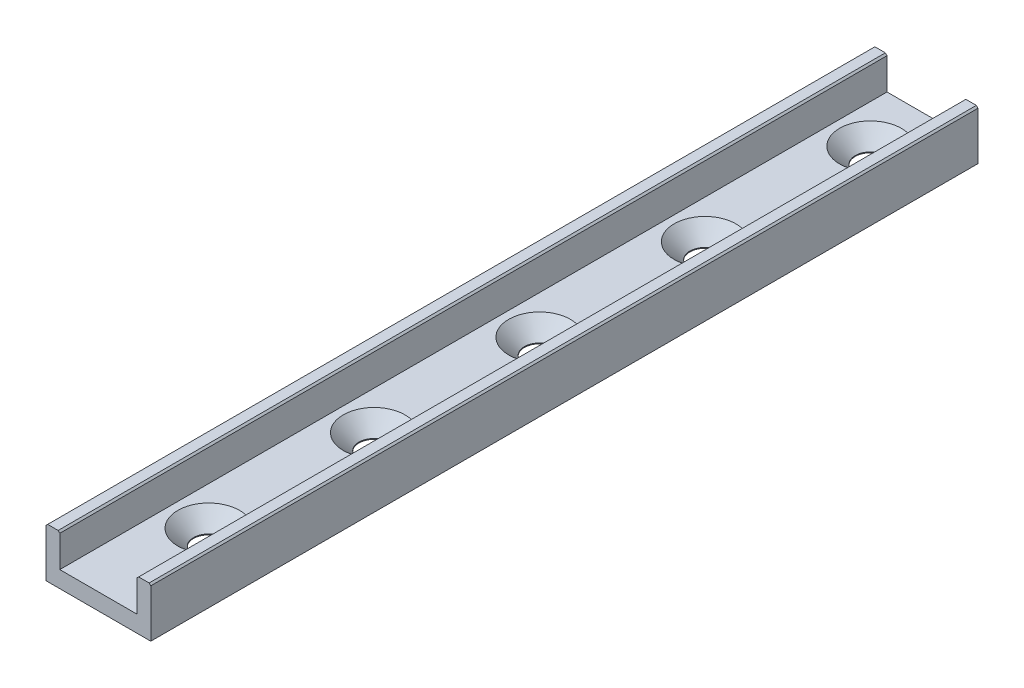
SolidWorks part; units mm, degrees
ref_plane "Front Plane" through (0, 0, 0) normal (0, 0, 1) x (1, 0, 0)
ref_plane "Top Plane" through (0, 0, 0) normal (0, 1, 0) x (1, 0, 0)
ref_plane "Right Plane" through (0, 0, 0) normal (1, 0, 0) x (0, 0, -1)
sketch "Sketch1" plane through (0, 0, 0) normal (0, 0, 1) x (1, 0, 0)
  line L0 (-7, 4.5) -> (-7, -1.5)
  line L1 (-9.5, -4.5) -> (9.5, -4.5)
  line L2 (-9.5, -4.5) -> (-9.5, 4.5)
  line L3 (-9.5, 4.5) -> (-7, 4.5)
  line L4 (9.5, -4.5) -> (9.5, 4.5)
  line L5 (-9.5, -4.5) -> (9.5, 4.5) construction
  line L6 (-9.5, 4.5) -> (9.5, -4.5) construction
  line L7 (-7, -1.5) -> (7, -1.5)
  line L8 (7, -1.5) -> (7, 4.5)
  line L9 (7, 4.5) -> (9.5, 4.5)
  point P0 (0, 0)
  dimension "D1" = 2.5
  dimension "D2" = 2.5
  dimension "D3" = 3
  dimension "D4" = 9
  dimension "D5" = 14
extrude "Boss-Extrude1" add sketch "Sketch1" along normal blind 150
hole_wizard "Hole size per Phillips slotted countersunk wood screw type 1" positions "Sketch4" profile "Sketch5" countersink size "M5" standard "GB" end condition through all
sketch "Sketch4" plane through (0, -1.5, 0) normal (0, 1, 0) x (1, 0, 0)
  line L0 (7, 0) -> (-7, 0) construction
  point P0 (0, -10)
  point P6 (0, -40)
  dimension "D1" = 10
  dimension "D2" = 30
sketch "Sketch5" plane through (0, -1.5, 10) normal (1, 0, 0) x (0, 0, 1)
  line L0 (0, 0) -> (0, 3)
  line L1 (0, 3) -> (2.75, 3)
  line L2 (2.75, 3) -> (2.75, 2.85)
  line L3 (2.75, 2.85) -> (5.6, 0)
  line L5 (5.6, 0) -> (0, 0)
  line L6 (-2.75, 2.85) -> (-5.6, 0) construction
  line L11 (0, -6.35) -> (0, 107.95) construction
  dimension "通孔孔直径" = 5.5
  dimension "通孔孔深度" = 3
  dimension "近端锥形沉头孔直径" = 11.2
  dimension "近端锥形沉头孔角度" = 90
pattern_linear "LPattern1" count 4 spacing 30 along (0, 0, 1) of "Hole size per Phillips slotted countersunk wood screw type 1"
chamfer "Chamfer1" distance 0.3 angle 45 4 edges at (-9.5, 4.5, 75) (9.5, 4.5, 75) (-7, 4.5, 75) (7, 4.5, 75)
